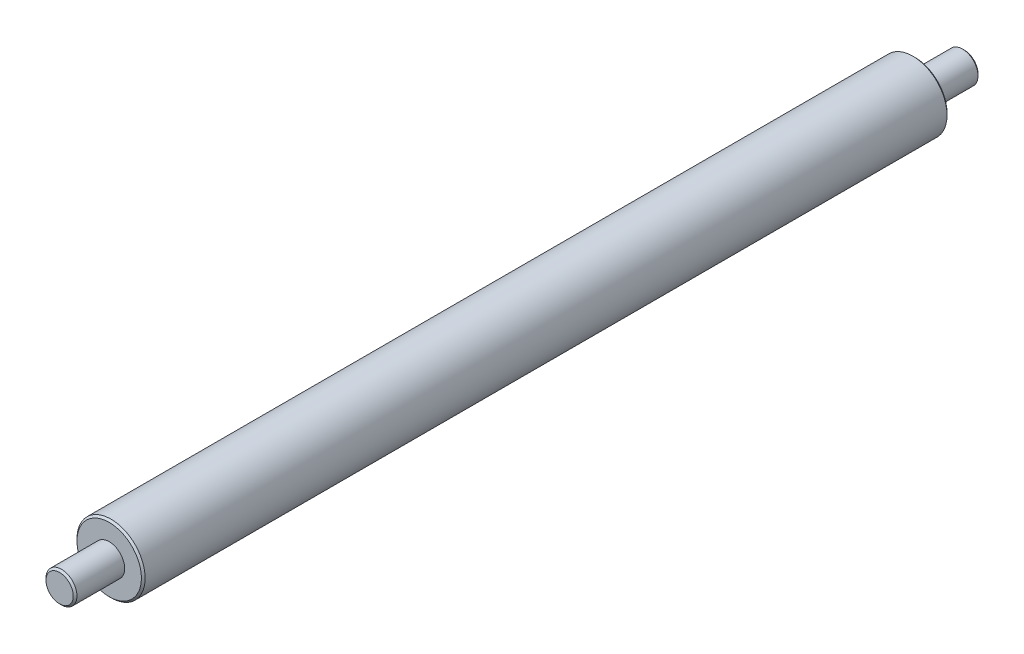
from build123d import *

# Parameters (mm, degrees)
SKETCH1_R           = 27.5
BOSS_EXTRUDE1_DEPTH = 325
SKETCH2_R           = 12.5
BOSS_EXTRUDE2_DEPTH = 40
CHAMFER1_SIZE       = 1.5


with BuildPart() as part:
    # Sketch1 → Boss-Extrude1 (new, symmetric)
    with BuildSketch(Plane.XY):
        Circle(SKETCH1_R)
    extrude(amount=BOSS_EXTRUDE1_DEPTH, both=True)

    # Sketch2 → Boss-Extrude2 (add)
    with BuildSketch(Plane.XY.offset(325)):
        Circle(SKETCH2_R)
    boss_extrude2 = extrude(amount=BOSS_EXTRUDE2_DEPTH)

    # Mirror1: Boss-Extrude2 across plane
    add(boss_extrude2.mirror(Plane.XY))

    # Chamfer1
    chamfer1_edges = [part.edges().sort_by_distance(p)[0] for p in [
        (-12.5, 0, -365),
        (-27.5, 0, -325),
        (-27.5, 0, 325),
        (-12.5, 0, 365),
    ]]
    chamfer(chamfer1_edges, length=CHAMFER1_SIZE)


solid = part.part
